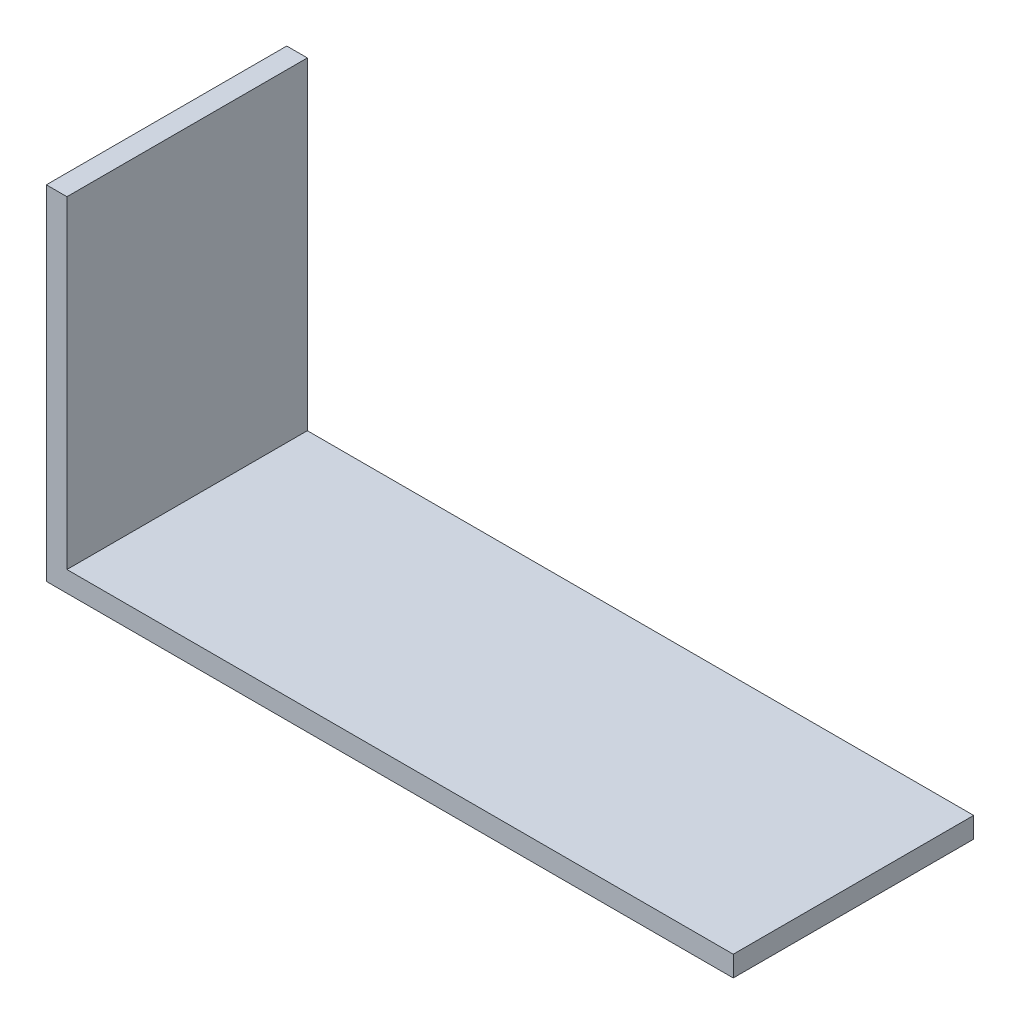
from build123d import *

# Parameters (mm, degrees)
EXTRUDE_1_DEPTH = 70


with BuildPart() as part:
    # 草图1 → 凸台-拉伸1 (new body)
    with BuildSketch(Plane.XY):
        Polygon((0, 0), (0, -100), (200, -100), (200, -94), (6, -94), (6, 0), align=None)
    extrude(amount=EXTRUDE_1_DEPTH)


solid = part.part
